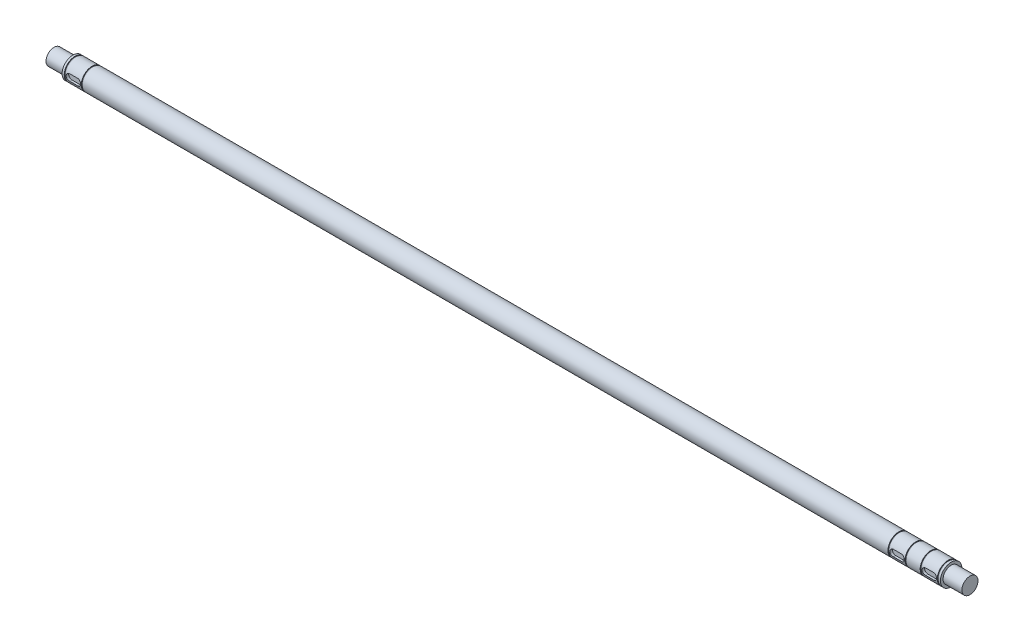
from build123d import *

# Parameters (mm, degrees)
SKETCH_1_R             = 20
EXTRUDE_1_DEPTH        = 1635.36
SKETCH_2_R             = 15
EXTRUDE_2_DEPTH        = 35
EXTRUDE_START          = 35
SKETCH_3_R             = 15
EXTRUDE_3_DEPTH        = 35
CUT_EXTRUDE_1_DEPTH    = 1671.846351284
SKETCH_5_W             = 1.85
SKETCH_5_H             = 1.25
SKETCH_7_W             = 1.85
SKETCH_7_H             = 1.25
PATTERN_LINEAR_2_COUNT = 2
PATTERN_LINEAR_2_PITCH = 60


with BuildPart() as part:
    # 草图1 → 凸台-拉伸1 (new body)
    with BuildSketch(Plane(origin=(0, 0, 0), x_dir=(0, 0, -1), z_dir=(1, 0, 0))):
        Circle(SKETCH_1_R)
    extrude(amount=EXTRUDE_1_DEPTH)

    # 草图2 → 凸台-拉伸2 (add)
    with BuildSketch(Plane.ZY):
        Circle(SKETCH_2_R)
    extrude(amount=EXTRUDE_2_DEPTH)

    # 草图3 → 凸台-拉伸3 (add)
    with BuildSketch(Plane(origin=(1635.36, 0, 0), x_dir=(0, 0, -1), z_dir=(1, 0, 0)).offset(EXTRUDE_START)):
        with Locations(Location((0, 0, 0), (0, 0, 180))):
            Circle(SKETCH_3_R)
    extrude(amount=-EXTRUDE_3_DEPTH)

    # 草图4 → 切除-拉伸1 (cut, through all)
    with BuildSketch(Plane.XY.offset(15)):
        with BuildLine():
            Line((13.3, 6), (28.3, 6))
            ThreePointArc((28.3, 6), (34.3, 0), (28.3, -6))
            Line((28.3, -6), (13.3, -6))
            ThreePointArc((13.3, -6), (7.3, 0), (13.3, 6))
        make_face()
        with BuildLine():
            Line((1622.06, -6), (1607.06, -6))
            ThreePointArc((1607.06, -6), (1601.06, 0), (1607.06, 6))
            Line((1607.06, 6), (1622.06, 6))
            ThreePointArc((1622.06, 6), (1628.06, 0), (1622.06, -6))
        make_face()
        with BuildLine():
            Line((1562.06, -6), (1547.06, -6))
            ThreePointArc((1547.06, -6), (1541.06, 0), (1547.06, 6))
            Line((1547.06, 6), (1562.06, 6))
            ThreePointArc((1562.06, 6), (1568.06, 0), (1562.06, -6))
        make_face()
    extrude(amount=CUT_EXTRUDE_1_DEPTH, mode=Mode.SUBTRACT)

    # 草图5 → 切除-旋转1 (revolve, cut)
    with BuildSketch(Plane.XY, mode=Mode.PRIVATE) as cut_revolve_1_sk:
        with Locations((4.875, 19.375)):
            Rectangle(SKETCH_5_W, SKETCH_5_H)
        with Locations((36.725, 19.375)):
            Rectangle(SKETCH_5_W, SKETCH_5_H)
    revolve(cut_revolve_1_sk.sketch.rotate(Axis((0, 0, 0), (1, 0, 0)), 90), axis=Axis((0, 0, 0), (1, 0, 0)), mode=Mode.SUBTRACT)

    # 草图7 → 切除-旋转2 (revolve, cut)
    with BuildSketch(Plane.XY, mode=Mode.PRIVATE) as cut_revolve_2_sk:
        with Locations((1598.635, 19.375)):
            Rectangle(SKETCH_7_W, SKETCH_7_H)
        with Locations((1630.485, 19.375)):
            Rectangle(SKETCH_7_W, SKETCH_7_H)
    cut_revolve_2 = revolve(cut_revolve_2_sk.sketch.rotate(Axis((1670.36, 0, 0), (-1, 0, 0)), 270), axis=Axis((1670.36, 0, 0), (-1, 0, 0)), mode=Mode.SUBTRACT)

    # 阵列(线性)2: 切除-旋转2 ×2
    with Locations(*[(-i * PATTERN_LINEAR_2_PITCH, 0, 0) for i in range(1, PATTERN_LINEAR_2_COUNT)]):
        add(cut_revolve_2, mode=Mode.SUBTRACT)


solid = part.part
